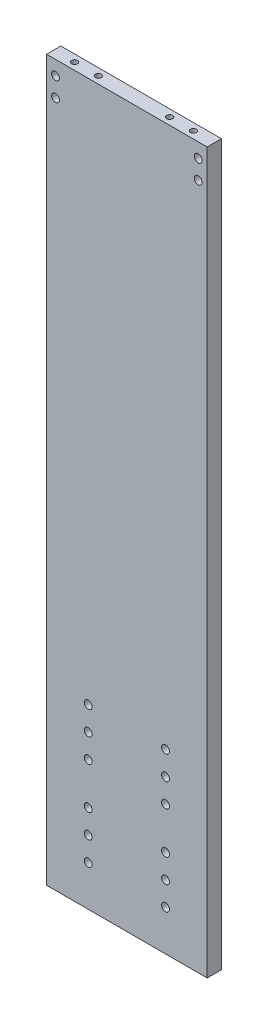
SolidWorks part; units mm, degrees
material "A6061"
ref_plane "前视基准面" through (0, 0, 0) normal (0, 0, 1) x (1, 0, 0)
ref_plane "上视基准面" through (0, 0, 0) normal (0, 1, 0) x (1, 0, 0)
ref_plane "右视基准面" through (0, 0, 0) normal (1, 0, 0) x (0, 0, -1)
sketch "草图1" plane through (0, 0, 0) normal (0, 0, 1) x (1, 0, 0)
  line L1 (-67.5, 302.5) -> (67.5, 302.5)
  line L2 (-67.5, 302.5) -> (-67.5, -302.5)
  line L3 (-67.5, -302.5) -> (67.5, -302.5)
  line L4 (67.5, 302.5) -> (67.5, -302.5)
  line L5 (-67.5, 302.5) -> (67.5, -302.5) construction
  line L6 (-67.5, -302.5) -> (67.5, 302.5) construction
  point P0 (0, 0)
  dimension "D1" = 605
  dimension "D2" = 135
extrude "凸台-拉伸1" add sketch "草图1" along normal mid plane 12
hole_wizard "M6 螺纹孔1" positions "草图2" profile "草图3" tap size "M6" standard "GB"
sketch "草图2" plane through (0, 302.5, 0) normal (0, 1, 0) x (1, 0, 0)
  line L0 (-67.5, 0) -> (50, 0) construction
  line L1 (-67.5, -6) -> (-67.5, 6) construction
  line L7 (0, 6) -> (0, -74.9797) construction
  line L8 (67.5, 6) -> (-67.5, 6) construction
  line L10 (67.5, 0) -> (-50, 0) construction
  point P0 (50, 0)
  point P38 (-30, 0)
  point P49 (30, 0)
  point P50 (-405, -6)
  point P55 (-50, 0)
  dimension "D1" = 60
  dimension "D2" = 20
cosmetic thread "孔螺蚊线1" parameters "D1"=12, "D2"=6
cosmetic thread "孔螺蚊线2" parameters "D1"=12, "D2"=6
cosmetic thread "孔螺蚊线3" parameters "D1"=12, "D2"=6
cosmetic thread "孔螺蚊线4" parameters "D1"=12, "D2"=6
sketch "草图3" plane through (50, 302.5, 0) normal (1, 0, 0) x (0, 0, 1)
  line L0 (0, 0) -> (0, 18.5022)
  line L1 (0, 18.5022) -> (2.5, 17)
  line L2 (2.5, 17) -> (2.5, 0)
  line L5 (2.5, 0) -> (0, 0)
  line L10 (0, 18.5022) -> (-2.5, 17) construction
  line L11 (0, -6.35) -> (0, 107.95) construction
  dimension "螺纹孔钻头直径" = 5
  dimension "螺纹孔钻头深度" = 17
  dimension "导头角度" = 118
hole_wizard "打孔尺寸(%根据)内六角圆柱头螺钉的类型2" positions "草图5" profile "草图6" counterbore size "M6" standard "GB" end condition through all
sketch "草图5" plane through (0, 0, -6) normal (0, 0, -1) x (-1, 0, 0)
  line L0 (0, 0) -> (0, 187.2441) construction
  line L2 (-67.5, 302.5) -> (67.5, 302.5) construction
  point P0 (-60, 290.5)
  point P2 (60, 290.5)
  point P17 (-60, 274.5)
  point P18 (60, 274.5)
  dimension "D1" = 120
  dimension "D2" = 12
  dimension "D4" = 16
  dimension "D3" = 2
sketch "草图6" plane through (60, 290.5, -6) normal (1, 0, 0) x (0, 1, 0)
  line L0 (0, 0) -> (0, 12)
  line L1 (0, 12) -> (3.3, 12)
  line L3 (3.3, 12) -> (3.3, 6.8)
  line L4 (3.3, 6.8) -> (5.5, 6.8)
  line L5 (5.5, 6.8) -> (5.5, 0)
  line L7 (5.5, 0) -> (0, 0)
  line L11 (0, -6.35) -> (0, 107.95) construction
  dimension "通孔孔直径" = 6.6
  dimension "通孔孔深度" = 12
  dimension "柱形沉头孔直径" = 11
  dimension "柱形沉头孔深度" = 6.8
hole_wizard "打孔尺寸(%根据)内六角圆柱头螺钉的类型2" positions "草图7" profile "草图8" counterbore size "M6" standard "GB" end condition through all
sketch "草图7" plane through (0, 0, -6) normal (0, 0, -1) x (-1, 0, 0)
  line L0 (0, -10.0378) -> (0, -259.273) construction
  line L2 (67.5, -302.5) -> (-67.5, -302.5) construction
  point P0 (-32.5, -153.5)
  point P3 (-32.5, -228.5)
  point P20 (32.5, -228.5)
  point P21 (32.5, -153.5)
  point P24 (32.5, -173.5)
  point P26 (32.5, -248.5)
  point P29 (-32.5, -248.5)
  point P30 (-32.5, -173.5)
  point P34 (32.5, -268.5)
  point P37 (32.5, -193.5)
  point P40 (-32.5, -193.5)
  point P41 (-32.5, -268.5)
sketch "草图8" plane through (32.5, -153.5, -6) normal (1, 0, 0) x (0, 1, 0)
  line L0 (0, 0) -> (0, 12)
  line L1 (0, 12) -> (3.3, 12)
  line L3 (3.3, 12) -> (3.3, 6.8)
  line L4 (3.3, 6.8) -> (5.5, 6.8)
  line L5 (5.5, 6.8) -> (5.5, 0)
  line L7 (5.5, 0) -> (0, 0)
  line L11 (0, -6.35) -> (0, 107.95) construction
  dimension "通孔孔直径" = 6.6
  dimension "通孔孔深度" = 12
  dimension "柱形沉头孔直径" = 11
  dimension "柱形沉头孔深度" = 6.8
equation "\"D6@草图7\"=\"D4@草图7\""
